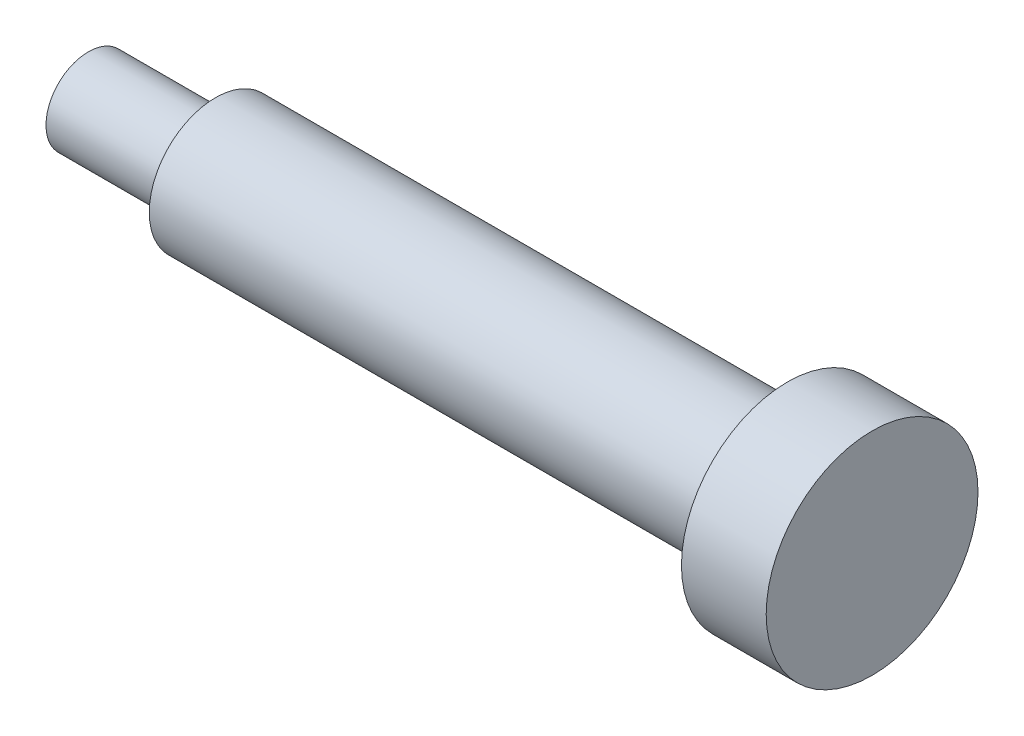
SolidWorks part; units mm, degrees
ref_plane "Front Plane" through (0, 0, 0) normal (0, 0, 1) x (1, 0, 0)
ref_plane "Top Plane" through (0, 0, 0) normal (0, 1, 0) x (1, 0, 0)
ref_plane "Right Plane" through (0, 0, 0) normal (1, 0, 0) x (0, 0, -1)
sketch "Sketch1" plane through (0, 0, 0) normal (0, 0, 1) x (1, 0, 0)
  line L0 (-26.6412, 0) -> (26.0133, 0) construction
  line L1 (-17.7608, 0) -> (-17.7608, -2)
  line L2 (-17.7608, -2) -> (-11.7608, -2)
  line L3 (-11.7608, -2) -> (-11.7608, -3.125)
  line L4 (-11.7608, -3.125) -> (15.2392, -3.125)
  line L5 (15.2392, -3.125) -> (15.2392, -5)
  line L6 (15.2392, -5) -> (19.2392, -5)
  line L7 (19.2392, -5) -> (19.2392, 0)
  line L8 (-17.7608, 0) -> (19.2392, 0)
  dimension "D1" = 27
  dimension "D2" = 4
  dimension "D3" = 37
  dimension "D4" = 2
  dimension "D5" = 3.125
  dimension "D6" = 5
revolve "Revolve1" add sketch "Sketch1" angle 360 about L0
